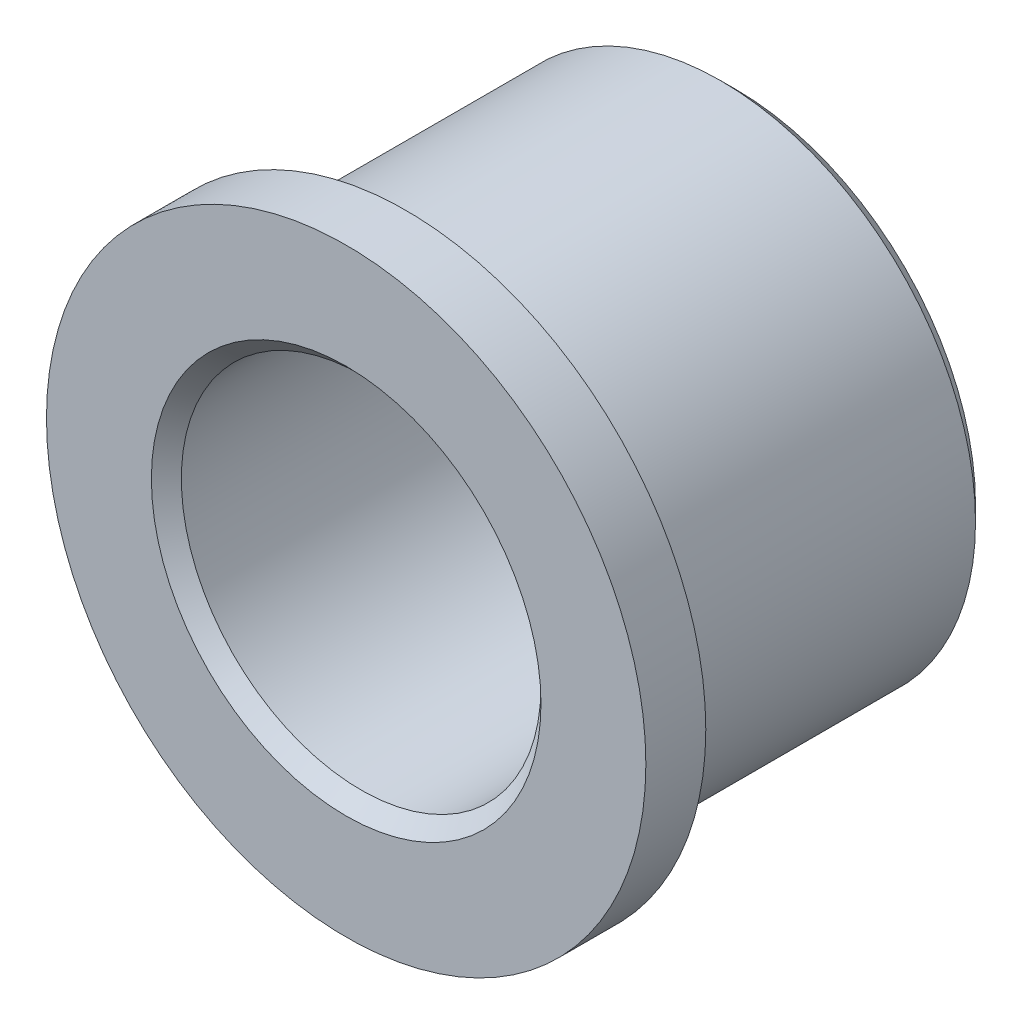
from build123d import *

# Parameters (mm, degrees)
SKETCH1_R           = 8.5
BOSS_EXTRUDE1_DEPTH = 13
SKETCH2_R           = 10
BOSS_EXTRUDE2_DEPTH = 2
SKETCH3_R           = 6
CUT_EXTRUDE1_DEPTH  = 25
CHAMFER1_SIZE       = 0.5


with BuildPart() as part:
    # Sketch1 → Boss-Extrude1 (new body)
    with BuildSketch(Plane.XY):
        with Locations(Location((0, 0, 0), (0, 0, 180))):
            Circle(SKETCH1_R)
    extrude(amount=BOSS_EXTRUDE1_DEPTH)

    # Sketch2 → Boss-Extrude2 (add)
    with BuildSketch(Plane.XY.offset(13)):
        Circle(SKETCH2_R)
    extrude(amount=-BOSS_EXTRUDE2_DEPTH)

    # Sketch3 → Cut-Extrude1 (cut)
    with BuildSketch(Plane(origin=(0, 0, 0), x_dir=(-1, 0, 0), z_dir=(0, 0, -1))):
        Circle(SKETCH3_R)
    extrude(amount=-CUT_EXTRUDE1_DEPTH, mode=Mode.SUBTRACT)

    # Chamfer1
    chamfer1_edges = [part.edges().sort_by_distance(p)[0] for p in [
        (6, 0, 13),
        (6, 0, 0),
        (8.5, 0, 0),
    ]]
    chamfer(chamfer1_edges, length=CHAMFER1_SIZE)


solid = part.part
